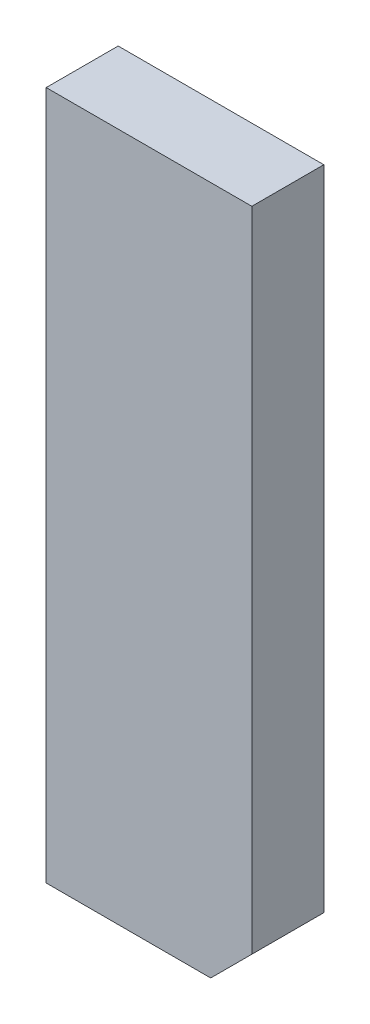
from build123d import *

# Parameters (mm, degrees)
SKETCH1_W           = 100
SKETCH1_H           = 335
BOSS_EXTRUDE1_DEPTH = 35
CHAMFER1_SIZE       = 20


with BuildPart() as part:
    # Sketch1 → Boss-Extrude1 (new body)
    with BuildSketch(Plane.XY):
        with Locations((50, -167.5)):
            Rectangle(SKETCH1_W, SKETCH1_H)
    extrude(amount=BOSS_EXTRUDE1_DEPTH)

    # Chamfer1
    chamfer1_edges = [part.edges().sort_by_distance(p)[0] for p in [
        (100, -335, 17.5),
    ]]
    chamfer(chamfer1_edges, length=CHAMFER1_SIZE)


solid = part.part
